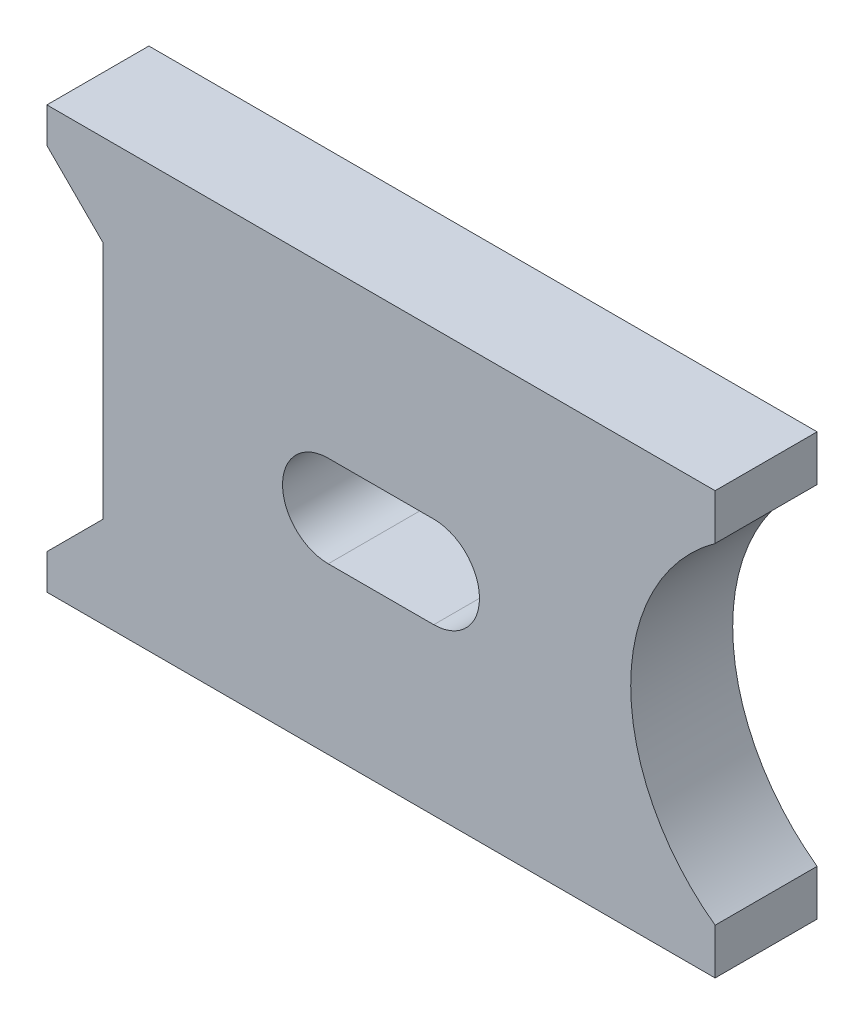
from build123d import *

# Parameters (mm, degrees)
BOSS_EXTRUDE1_DEPTH = 14.5


with BuildPart() as part:
    # Sketch1 → Boss-Extrude1 (new body)
    with BuildSketch(Plane.XY):
        with BuildLine():
            ThreePointArc((47.5, 23.5), (35.5, 0), (47.5, -23.5))
            Line((47.5, -23.5), (47.5, -30))
            Line((47.5, -30), (-47.5, -30))
            Line((-47.5, -30), (-47.5, -25))
            Line((-47.5, -25), (-39.5, -17))
            Line((-39.5, -17), (-39.5, 17))
            Line((-39.5, 17), (-47.5, 25))
            Line((-47.5, 25), (-47.5, 30))
            Line((-47.5, 30), (47.5, 30))
            Line((47.5, 30), (47.5, 23.5))
        make_face()
        with BuildLine():
            Line((-7.5, -6.5), (7.5, -6.5))
            ThreePointArc((7.5, -6.5), (14, 0), (7.5, 6.5))
            Line((7.5, 6.5), (-7.5, 6.5))
            ThreePointArc((-7.5, 6.5), (-14, 0), (-7.5, -6.5))
        make_face(mode=Mode.SUBTRACT)
    extrude(amount=BOSS_EXTRUDE1_DEPTH)


solid = part.part
